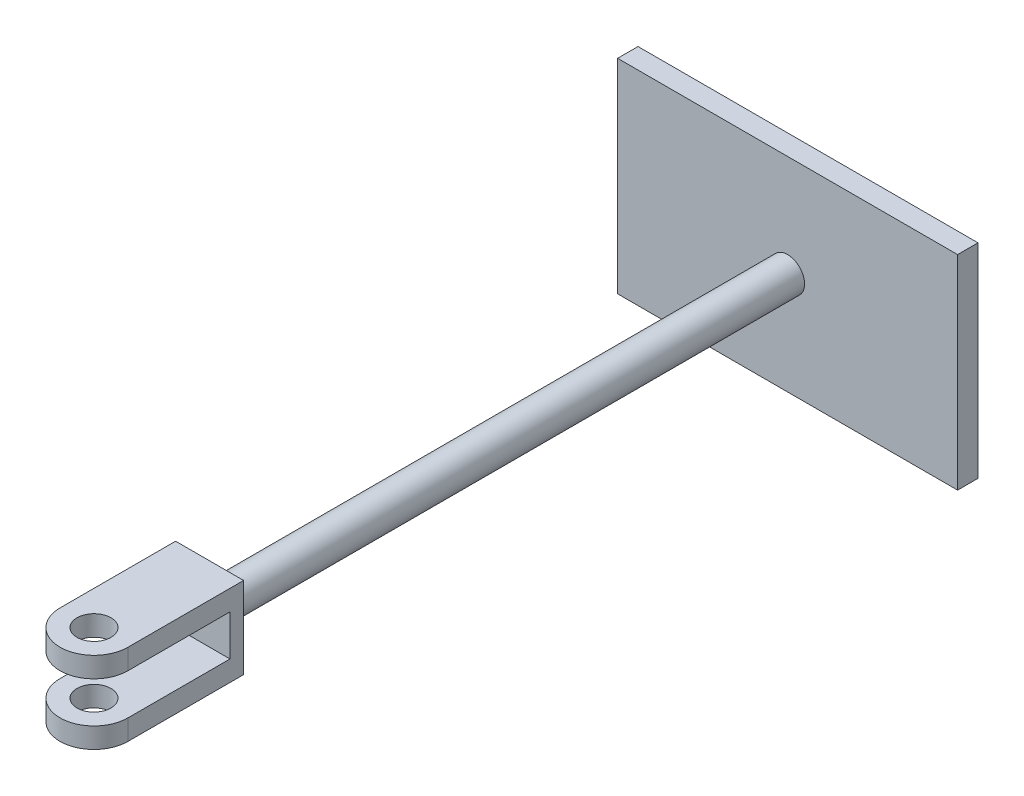
from build123d import *

# Parameters (mm, degrees)
SKETCH1_W           = 50
SKETCH1_H           = 30
BOSS_EXTRUDE1_DEPTH = 3
SKETCH2_R           = 2.5
BOSS_EXTRUDE2_DEPTH = 85
SKETCH3_W           = 10
SKETCH3_H           = 12
BOSS_EXTRUDE3_DEPTH = 22
SKETCH4_W           = 17.596186584
SKETCH4_H           = 6
CUT_EXTRUDE1_DEPTH  = 20
SKETCH5_R           = 2.5
CUT_EXTRUDE2_DEPTH  = 115.743191519


with BuildPart() as part:
    # Sketch1 → Boss-Extrude1 (new body)
    with BuildSketch(Plane.XY):
        Rectangle(SKETCH1_W, SKETCH1_H)
    extrude(amount=BOSS_EXTRUDE1_DEPTH)

    # Sketch2 → Boss-Extrude2 (add)
    with BuildSketch(Plane.XY.offset(3)):
        Circle(SKETCH2_R)
    extrude(amount=BOSS_EXTRUDE2_DEPTH)

    # Sketch3 → Boss-Extrude3 (add)
    with BuildSketch(Plane.XY.offset(88)):
        Rectangle(SKETCH3_W, SKETCH3_H)
    extrude(amount=BOSS_EXTRUDE3_DEPTH)

    # Sketch4 → Cut-Extrude1 (cut)
    with BuildSketch(Plane.XY.offset(110)):
        Rectangle(SKETCH4_W, SKETCH4_H)
    extrude(amount=-CUT_EXTRUDE1_DEPTH, mode=Mode.SUBTRACT)

    # Sketch5 → Cut-Extrude2 (cut, through all)
    with BuildSketch(Plane(origin=(0, -6, 0), x_dir=(-1, 0, 0), z_dir=(0, -1, 0))):
        with Locations(Location((0, -105, 0), (0, 0, 90))):
            Circle(SKETCH5_R)
        with BuildLine():
            Line((5, -105), (16.865416132, -140.325641039))
            Line((16.865416132, -140.325641039), (-16.120021854, -140.325641039))
            Line((-16.120021854, -140.325641039), (-5, -105))
            ThreePointArc((-5, -105), (0, -110), (5, -105))
        make_face()
    extrude(amount=-CUT_EXTRUDE2_DEPTH, mode=Mode.SUBTRACT)


solid = part.part
